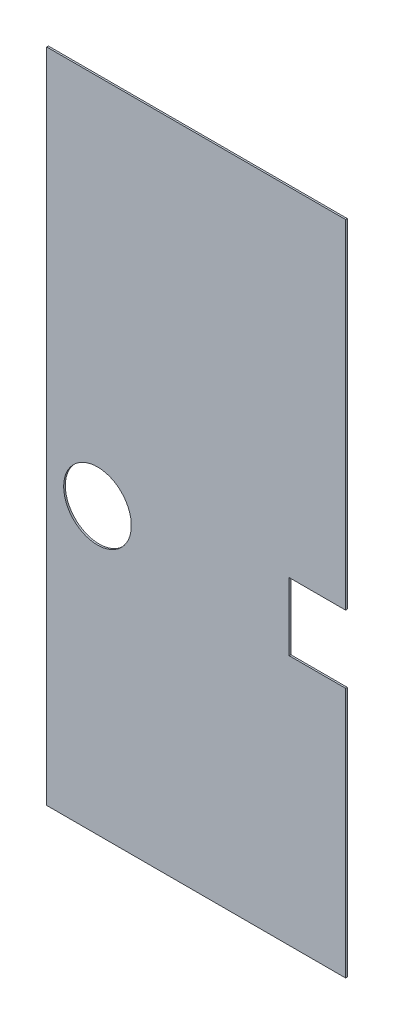
SolidWorks part; units mm, degrees
material "Q235"
ref_plane "Front Plane" through (0, 0, 0) normal (0, 0, 1) x (1, 0, 0)
ref_plane "Top Plane" through (0, 0, 0) normal (0, 1, 0) x (1, 0, 0)
ref_plane "Right Plane" through (0, 0, 0) normal (1, 0, 0) x (0, 0, -1)
sketch "Sketch1" plane through (0, 0, 0) normal (0, 0, 1) x (1, 0, 0)
  line L1 (0, 0) -> (530, 0)
  line L2 (0, 0) -> (0, 1165)
  line L3 (0, 1165) -> (530, 1165)
  line L4 (530, 0) -> (530, 1165)
  dimension "D1" = 530
  dimension "D2" = 1165
extrude "Boss-Extrude1" add sketch "Sketch1" along normal blind 3
sketch "Sketch2" plane through (0, 0, 0) normal (0, 0, -1) x (-1, 0, 0)
  line L0 (-530, 1165) -> (0, 1165) construction
  line L1 (-490, 505) -> (-90, 505) construction
  line L2 (-530, 0) -> (-530, 1165) construction
  line L4 (-430, 445) -> (-550, 445)
  line L5 (-430, 445) -> (-430, 565)
  line L6 (-430, 565) -> (-550, 565)
  line L7 (-550, 445) -> (-550, 565)
  line L8 (-430, 445) -> (-550, 565) construction
  line L9 (-430, 565) -> (-550, 445) construction
  circle A0 centre (-90, 505) radius 60
  circle A1 centre (-490, 505) radius 60 construction
  dimension "D1" = 120
  dimension "D2" = 120
  dimension "D4" = 40
  dimension "D3" = 660
  dimension "D5" = 400
extrude "Cut-Extrude1" cut sketch "Sketch2" against normal blind 10
